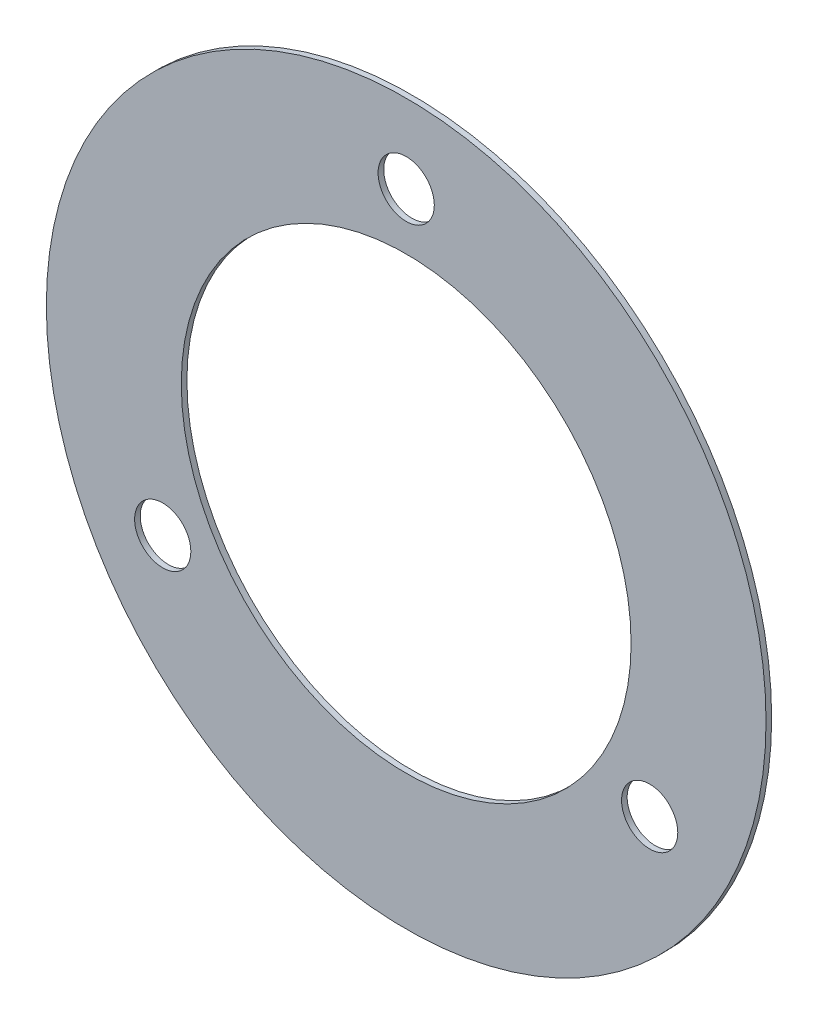
from build123d import *

# Parameters (mm, degrees)
SKETCH1_R           = 32
SKETCH1_R_2         = 20
BOSS_EXTRUDE1_DEPTH = 0.5
SKETCH2_R           = 2.5
CUT_EXTRUDE1_DEPTH  = 0.5


with BuildPart() as part:
    # Sketch1 → Boss-Extrude1 (new body)
    with BuildSketch(Plane.XY):
        Circle(SKETCH1_R)
        Circle(SKETCH1_R_2, mode=Mode.SUBTRACT)
    extrude(amount=BOSS_EXTRUDE1_DEPTH)

    # Sketch2 → Cut-Extrude1 (cut)
    with BuildSketch(Plane.XY.offset(0.5)):
        with Locations((0, 25)):
            Circle(SKETCH2_R)
        with Locations((21.650635095, -12.5)):
            Circle(SKETCH2_R)
        with Locations((-21.650635095, -12.5)):
            Circle(SKETCH2_R)
    extrude(amount=-CUT_EXTRUDE1_DEPTH, mode=Mode.SUBTRACT)


solid = part.part
